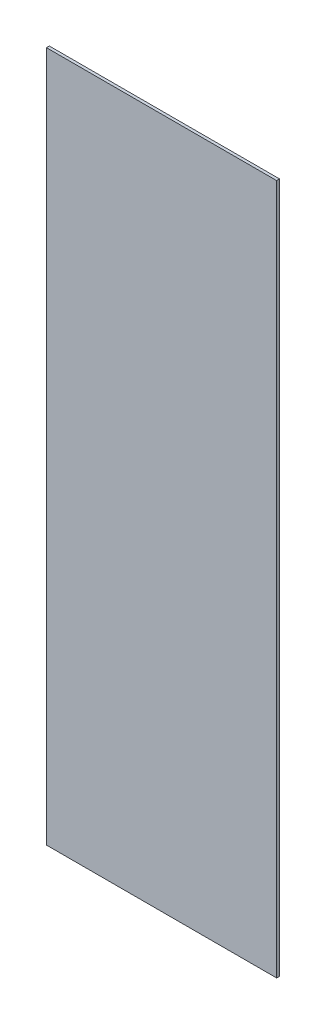
SolidWorks part; units mm, degrees
ref_plane "Front Plane" through (0, 0, 0) normal (0, 0, 1) x (1, 0, 0)
ref_plane "Top Plane" through (0, 0, 0) normal (0, 1, 0) x (1, 0, 0)
ref_plane "Right Plane" through (0, 0, 0) normal (1, 0, 0) x (0, 0, -1)
sketch "Sketch1" plane through (0, 0, 0) normal (0, 0, 1) x (1, 0, 0)
  line L1 (-40, 120) -> (40, 120)
  line L2 (-40, 120) -> (-40, -120)
  line L3 (-40, -120) -> (40, -120)
  line L4 (40, 120) -> (40, -120)
  line L5 (-40, 120) -> (40, -120) construction
  line L6 (-40, -120) -> (40, 120) construction
  point P0 (0, 0)
  dimension "D1" = 80
  dimension "D2" = 240
extrude "Boss-Extrude1" add sketch "Sketch1" along normal blind 1
